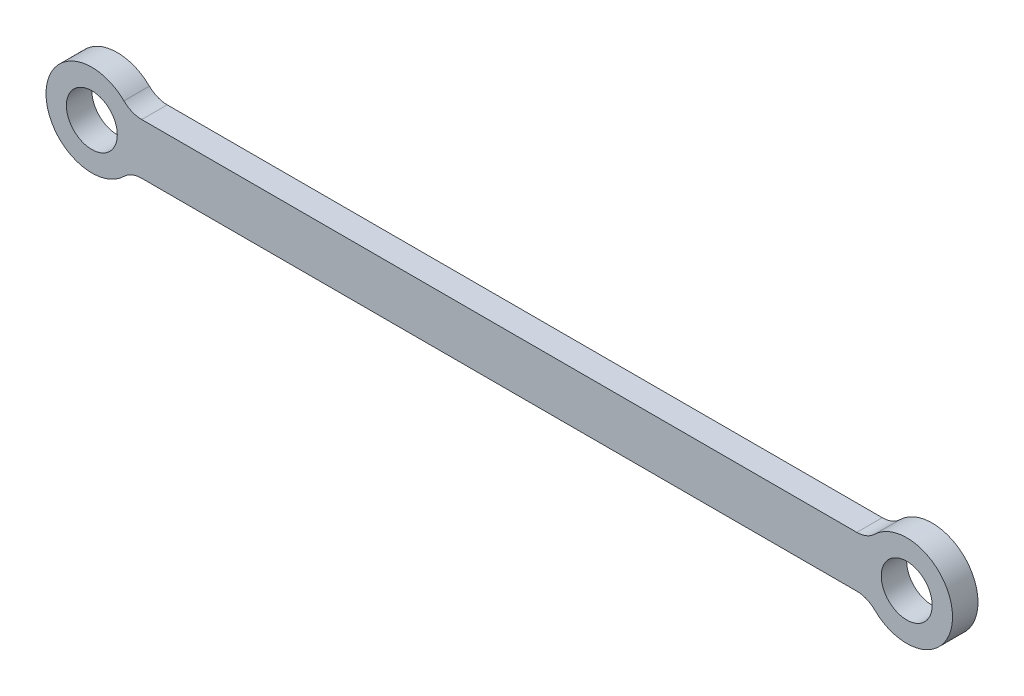
from build123d import *

# Parameters (mm, degrees)
SKETCH1_R           = 5
BOSS_EXTRUDE1_DEPTH = 5


with BuildPart() as part:
    # Sketch1 → Boss-Extrude1 (new body)
    with BuildSketch(Plane.XY):
        with BuildLine():
            Line((9.797958971, 5), (150.202041029, 5))
            ThreePointArc((150.202041029, 5), (152.091863394, 5.370899501), (153.70131209, 6.428571429))
            ThreePointArc((153.70131209, 6.428571429), (169, 0), (153.70131209, -6.428571429))
            ThreePointArc((153.70131209, -6.428571429), (152.091863394, -5.370899501), (150.202041029, -5))
            Line((150.202041029, -5), (9.797958971, -5))
            ThreePointArc((9.797958971, -5), (7.908136606, -5.370899501), (6.29868791, -6.428571429))
            ThreePointArc((6.29868791, -6.428571429), (-9, 0), (6.29868791, 6.428571429))
            ThreePointArc((6.29868791, 6.428571429), (7.908136606, 5.370899501), (9.797958971, 5))
        make_face()
        Circle(SKETCH1_R, mode=Mode.SUBTRACT)
        with Locations((160, 0)):
            Circle(SKETCH1_R, mode=Mode.SUBTRACT)
    extrude(amount=BOSS_EXTRUDE1_DEPTH)


solid = part.part
